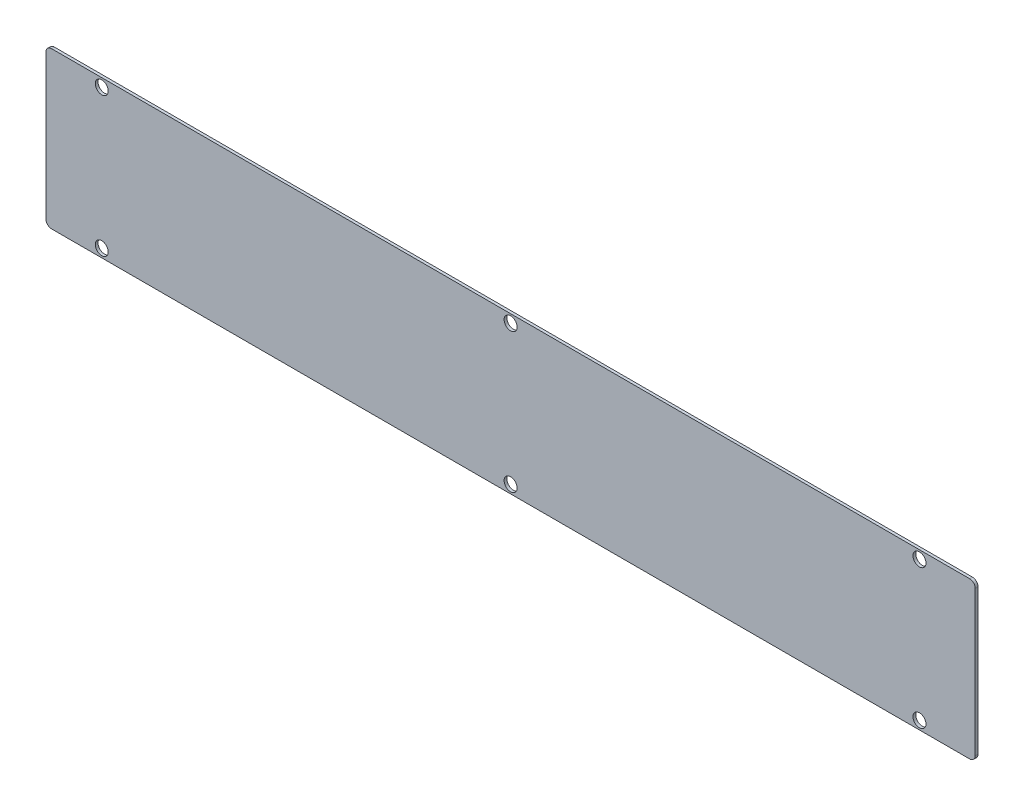
from build123d import *

# Parameters (mm, degrees)
SKETCH_1_W          = 500
SKETCH_1_H          = 84
EXTRUDE_1_DEPTH     = 1.5
SKETCH_2_R          = 3.5
CUT_EXTRUDE_1_DEPTH = 254.507889424
FILLET_1_R          = 3


with BuildPart() as part:
    # 草图1 → 凸台-拉伸1 (new body)
    with BuildSketch(Plane.XY):
        Rectangle(SKETCH_1_W, SKETCH_1_H)
    extrude(amount=EXTRUDE_1_DEPTH)

    # 草图2 → 切除-拉伸1 (cut, through all)
    with BuildSketch(Plane(origin=(0, 0, 0), x_dir=(-1, 0, 0), z_dir=(0, 0, -1))):
        with Locations(Location((0, 37.5, 0), (0, 0, 180))):
            Circle(SKETCH_2_R)
        with Locations(Location((220, 37.5, 0), (0, 0, 180))):
            Circle(SKETCH_2_R)
        with Locations((-220, -37.5)):
            Circle(SKETCH_2_R)
        with Locations((220, -37.5)):
            Circle(SKETCH_2_R)
        with Locations((0, -37.5)):
            Circle(SKETCH_2_R)
        with Locations(Location((-220, 37.5, 0), (0, 0, 180))):
            Circle(SKETCH_2_R)
    extrude(amount=-CUT_EXTRUDE_1_DEPTH, mode=Mode.SUBTRACT)

    # 圆角1
    fillet_1_edges = [part.edges().sort_by_distance(p)[0] for p in [
        (250, -42, 0.75),
        (-250, -42, 0.75),
        (-250, 42, 0.75),
        (250, 42, 0.75),
    ]]
    fillet(fillet_1_edges, radius=FILLET_1_R)


solid = part.part
